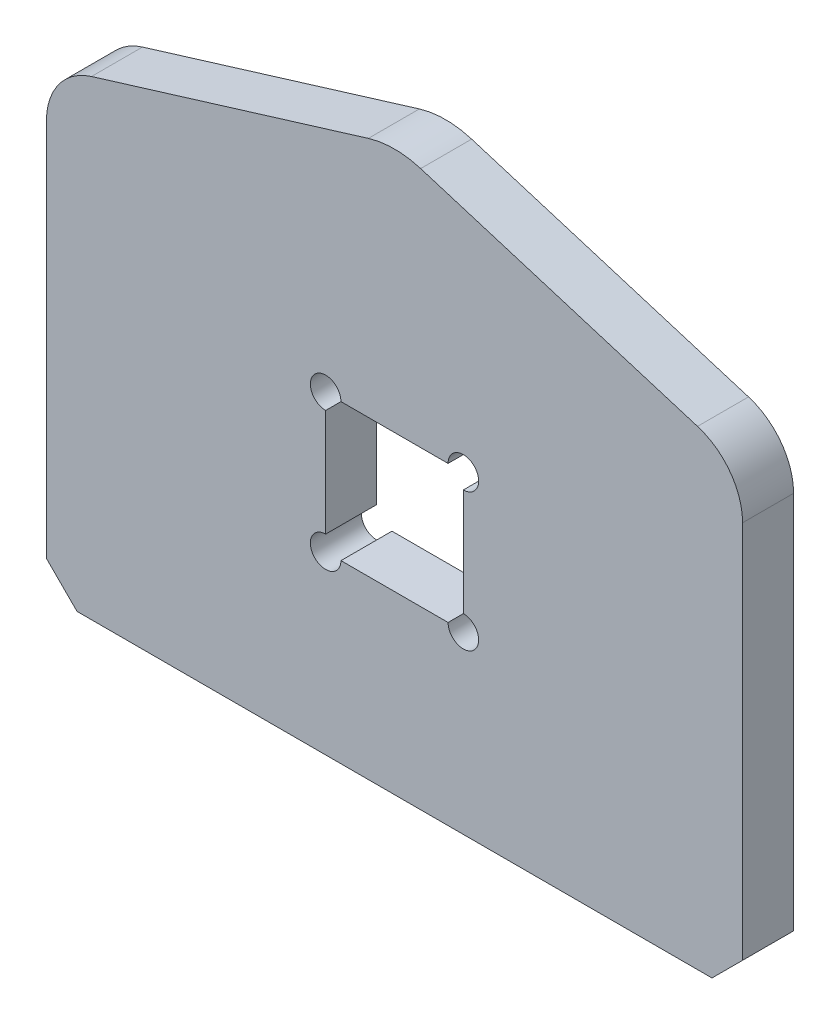
from build123d import *

# Parameters (mm, degrees)
BOSS_EXTRUDE1_DEPTH = 20


with BuildPart() as part:
    # Sketch1 → Boss-Extrude1 (new body)
    with BuildSketch(Plane.XY):
        with BuildLine():
            Line((-124.5, 0), (124.5, 0))
            Line((124.5, 0), (136.5, 12))
            Line((136.5, 12), (136.5, 160.6))
            ThreePointArc((136.5, 160.6), (131.600675284, 175.464819311), (118.822971749, 184.503432489))
            Line((118.822971749, 184.503432489), (10.252160448, 217.764805485))
            ThreePointArc((10.252160448, 217.764805485), (0, 219.3), (-10.252160448, 217.764805485))
            Line((-10.252160448, 217.764805485), (-118.822971749, 184.503432489))
            ThreePointArc((-118.822971749, 184.503432489), (-131.600675284, 175.464819311), (-136.5, 160.6))
            Line((-136.5, 160.6), (-136.5, 12))
            Line((-136.5, 12), (-124.5, 0))
        make_face()
        with BuildLine():
            Line((-21, 123), (21, 123))
            ThreePointArc((21, 123), (31.242640687, 127.242640687), (27, 117))
            Line((27, 117), (27, 75))
            ThreePointArc((27, 75), (31.242640687, 64.757359313), (21, 69))
            Line((21, 69), (-21, 69))
            ThreePointArc((-21, 69), (-31.242640687, 64.757359313), (-27, 75))
            Line((-27, 75), (-27, 117))
            ThreePointArc((-27, 117), (-31.242640687, 127.242640687), (-21, 123))
        make_face(mode=Mode.SUBTRACT)
    extrude(amount=BOSS_EXTRUDE1_DEPTH)


solid = part.part
